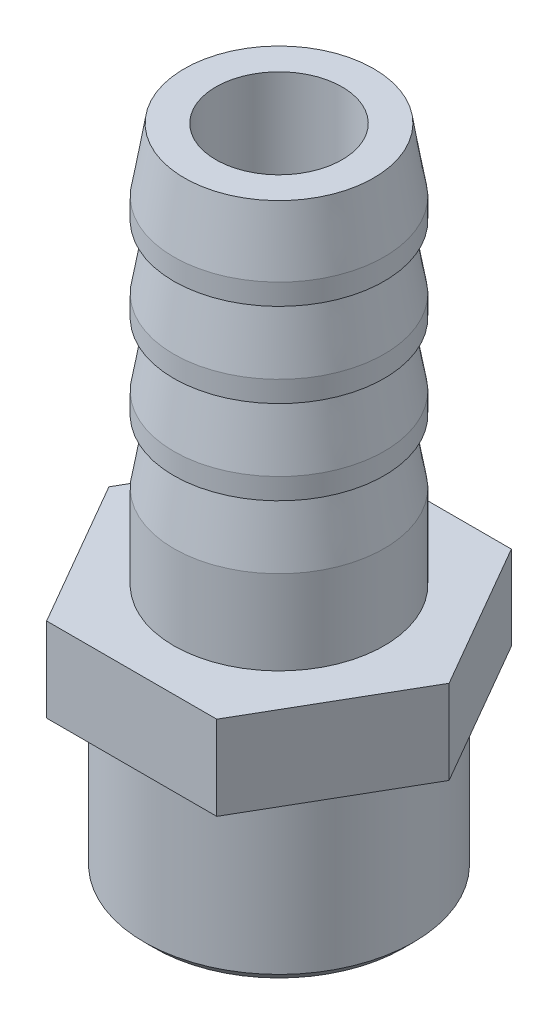
from build123d import *

# Parameters (mm, degrees)
EXTRUDE_1_DEPTH     = 4
SKETCH_3_R          = 6.4
EXTRUDE_2_DEPTH     = 8
CUT_EXTRUDE_1_REACH = 34.792
SKETCH_4_R          = 3
CHAMFER_1_SIZE      = 0.5


with BuildPart() as part:
    # 草图1 → 旋转1 (revolve)
    with BuildSketch(Plane.XY, mode=Mode.PRIVATE) as revolve_1_sk:
        Polygon((-5, 4), (-4.5, 7), (-5, 7), (-5, 8), (-4.5, 11), (-5, 11), (-5, 12), (-4.5, 15), (-5, 15), (-5, 16), (-4.5, 19), (0, 19), (0, 0), (-5, 0), align=None)
    revolve(revolve_1_sk.sketch.rotate(Axis((0, 0, 0), (0, 1, 0)), 270), axis=Axis((0, 0, 0), (0, 1, 0)))

    # 草图2 → 凸台-拉伸1 (add)
    with BuildSketch(Plane.XZ):
        Polygon((8.082903769, 0), (4.041451884, 7), (-4.041451884, 7), (-8.082903769, 0), (-4.041451884, -7), (4.041451884, -7), align=None)
    extrude(amount=EXTRUDE_1_DEPTH)

    # 草图3 → 凸台-拉伸2 (add)
    with BuildSketch(Plane.XZ.offset(4)):
        Circle(SKETCH_3_R)
    extrude(amount=EXTRUDE_2_DEPTH)

    # 草图4 → 切除-拉伸1 (cut, up to next)
    with BuildSketch(Plane(origin=(0, 19, 0), x_dir=(1, 0, 0), z_dir=(0, 1, 0)), mode=Mode.PRIVATE) as cut_extrude_1_sk1:
        with Locations(Location((0, 0, 0), (0, 0, 180))):
            Circle(SKETCH_4_R)
    cut_extrude_1_tool1 = extrude(cut_extrude_1_sk1.sketch, amount=-CUT_EXTRUDE_1_REACH, mode=Mode.PRIVATE) & part.part
    add(cut_extrude_1_tool1.solids().sort_by_distance((0, 19, 0))[0], mode=Mode.SUBTRACT)

    # 倒角1
    chamfer_1_edges = [part.edges().sort_by_distance(p)[0] for p in [
        (-6.4, -12, 0),
    ]]
    chamfer(chamfer_1_edges, length=CHAMFER_1_SIZE)


solid = part.part
